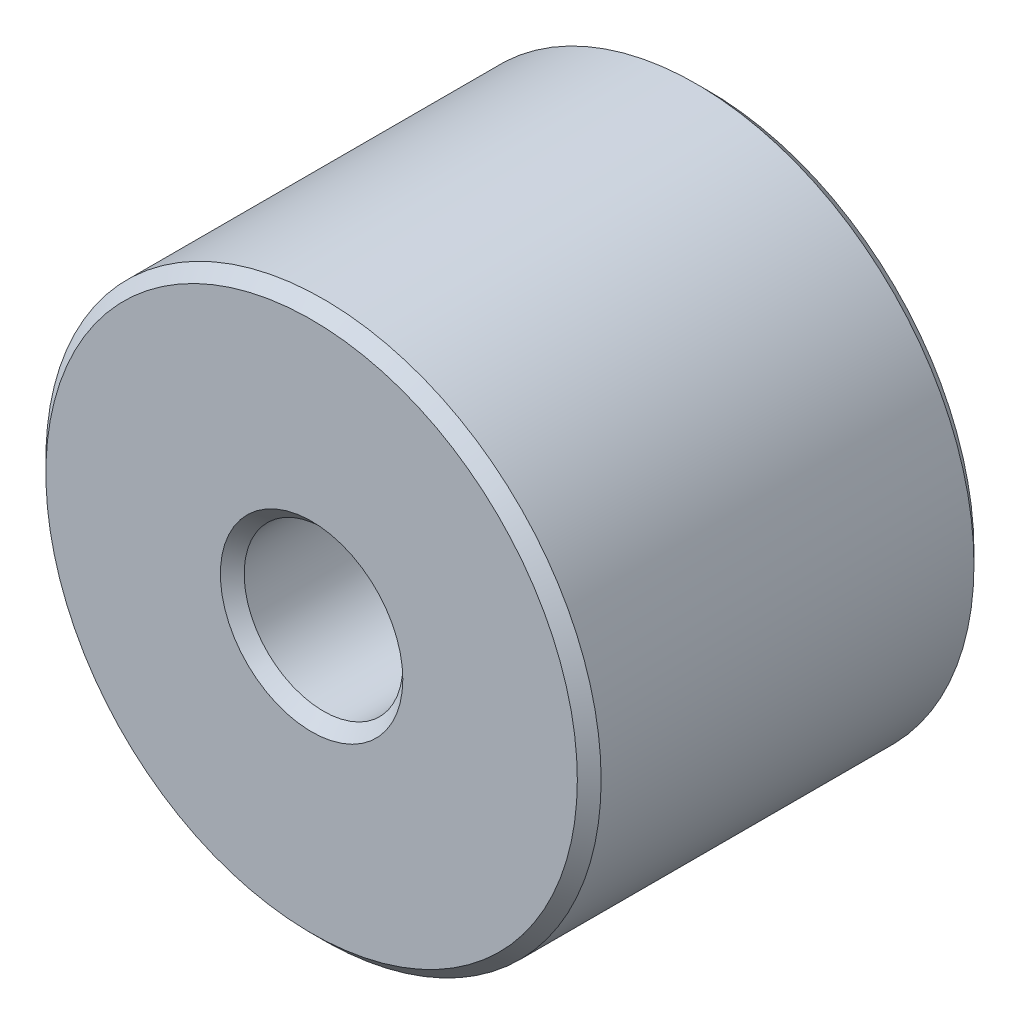
SolidWorks part; units mm, degrees
ref_plane "Front Plane" through (0, 0, 0) normal (0, 0, 1) x (1, 0, 0)
ref_plane "Top Plane" through (0, 0, 0) normal (0, 1, 0) x (1, 0, 0)
ref_plane "Right Plane" through (0, 0, 0) normal (1, 0, 0) x (0, 0, -1)
other "Configuration Table"
sketch "Sketch1" plane through (0, 0, 0) normal (0, 0, 1) x (1, 0, 0)
  circle A0 centre (0, 0) radius 3.6
  circle A1 centre (0, 0) radius 12.6
  dimension "D1" = 7.2
  dimension "D2" = 25.2
extrude "Boss-Extrude1" add sketch "Sketch1" along normal blind 18
chamfer "Chamfer1" distance 0.54 angle 45 4 edges at (3.6, 0, 18) (3.6, 0, 0) (12.6, 0, 0) (12.6, 0, 18)
